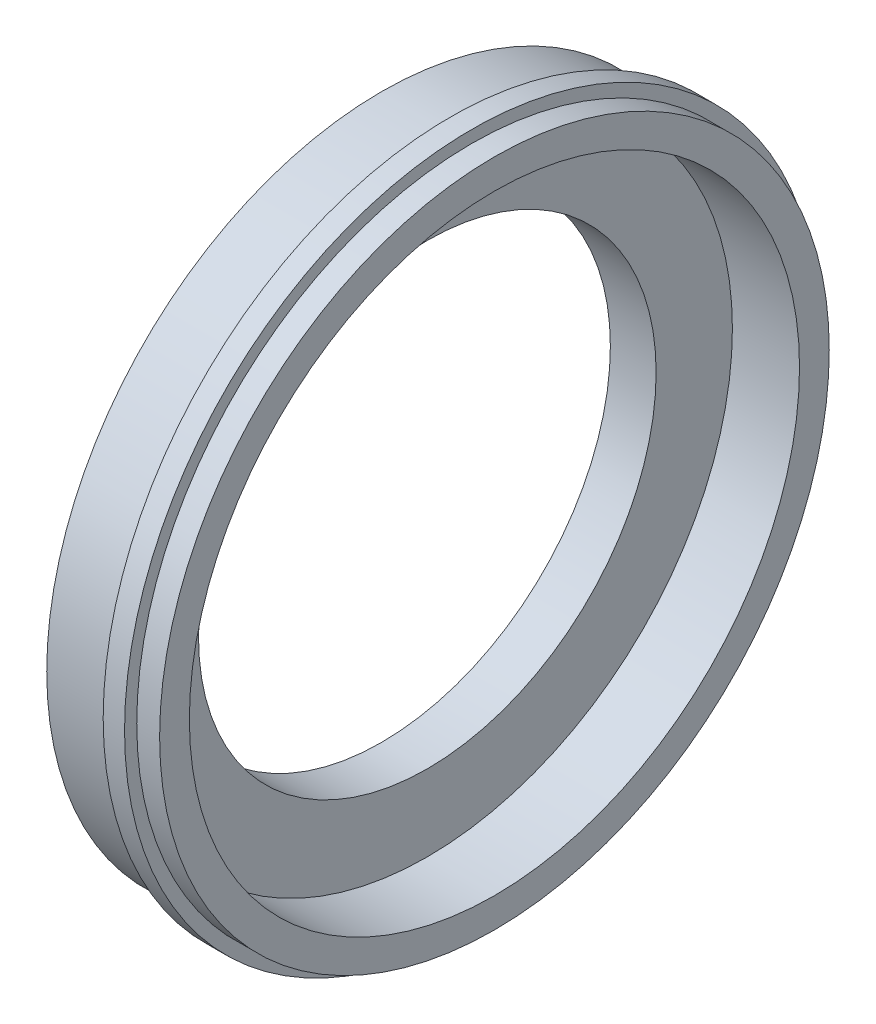
from build123d import *


with BuildPart() as part:
    # Sketch1 → Revolve1 (revolve)
    with BuildSketch(Plane(origin=(0, 0, 0), x_dir=(1, 0, 0), z_dir=(0, 1, 0)), mode=Mode.PRIVATE) as revolve1_sk:
        Polygon((0, 150), (0, 163), (14, 163), (14, 177), (0, 177), (0, 189), (14, 189), (14, 203), (0, 203), (0, 219.5), (45, 219.5), (45, 227.5), (59, 227.5), (59, 219.5), (74, 219.5), (74, 200), (30, 200), (30, 150), align=None)
    revolve(revolve1_sk.sketch.rotate(Axis((0, 0, 0), (1, 0, 0)), 180), axis=Axis((0, 0, 0), (1, 0, 0)))


solid = part.part
